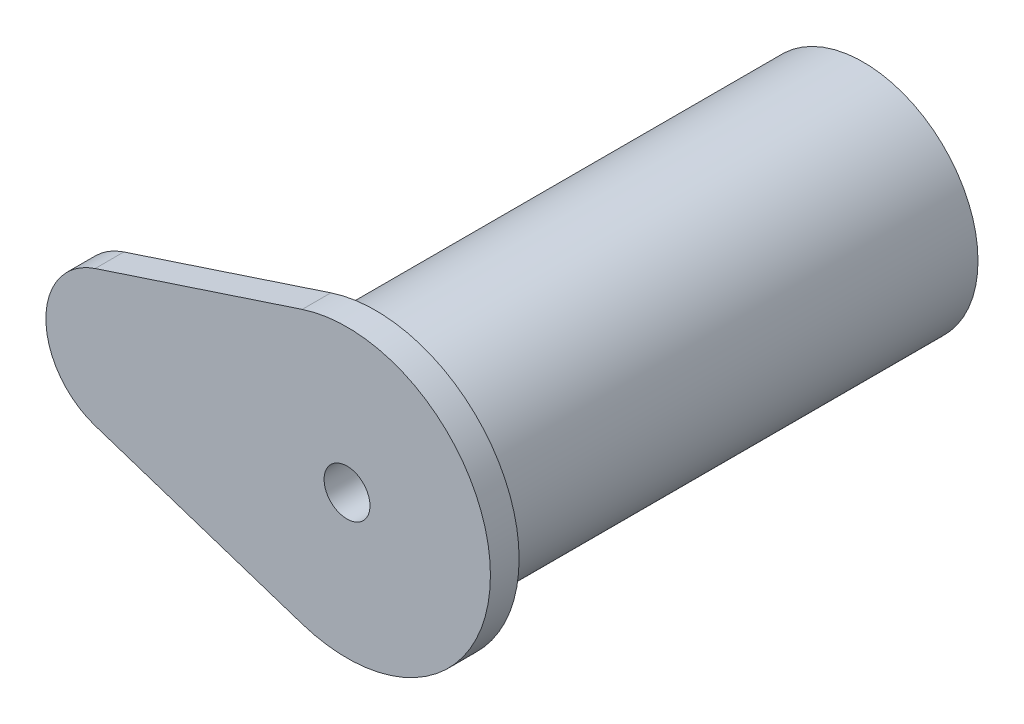
from build123d import *

# Parameters (mm, degrees)
SKETCH_1_R          = 20
EXTRUDE_1_DEPTH     = 90
EXTRUDE_2_DEPTH     = 5
SKETCH_3_R          = 4
CUT_EXTRUDE_1_DEPTH = 60
CUT_EXTRUDE_2_DEPTH = 20


with BuildPart() as part:
    # 草图1 → 凸台-拉伸1 (new body)
    with BuildSketch(Plane.XY):
        with Locations(Location((0, 0, 0), (0, 0, 180))):
            Circle(SKETCH_1_R)
    extrude(amount=EXTRUDE_1_DEPTH)

    # 草图2 → 凸台-拉伸2 (add)
    with BuildSketch(Plane.XY.offset(90)):
        with BuildLine():
            Line((-43.90625, 11.873971995), (-7.8125, 23.74794399))
            ThreePointArc((-7.8125, 23.74794399), (25, 0), (-7.8125, -23.74794399))
            Line((-7.8125, -23.74794399), (-43.90625, -11.873971995))
            ThreePointArc((-43.90625, -11.873971995), (-52.5, 0), (-43.90625, 11.873971995))
        make_face()
    extrude(amount=-EXTRUDE_2_DEPTH)

    # 草图3 → 切除-拉伸1 (cut)
    with BuildSketch(Plane.XY.offset(90)):
        Circle(SKETCH_3_R)
    extrude(amount=-CUT_EXTRUDE_1_DEPTH, mode=Mode.SUBTRACT)

    # 草图4 → 切除-拉伸2 (cut)
    with BuildSketch(Plane(origin=(0, 0, 0), x_dir=(1, 0, 0), z_dir=(0, 1, 0))):
        with BuildLine():
            ThreePointArc((4, -42.5), (2.828427125, -39.671572875), (0, -38.5))
            Line((0, -38.5), (0, -46.5))
            ThreePointArc((0, -46.5), (2.828427125, -45.328427125), (4, -42.5))
        make_face()
        with BuildLine():
            Line((0, -46.5), (0, -38.5))
            ThreePointArc((0, -38.5), (-4, -42.5), (0, -46.5))
        make_face()
    extrude(amount=-CUT_EXTRUDE_2_DEPTH, mode=Mode.SUBTRACT)


solid = part.part
